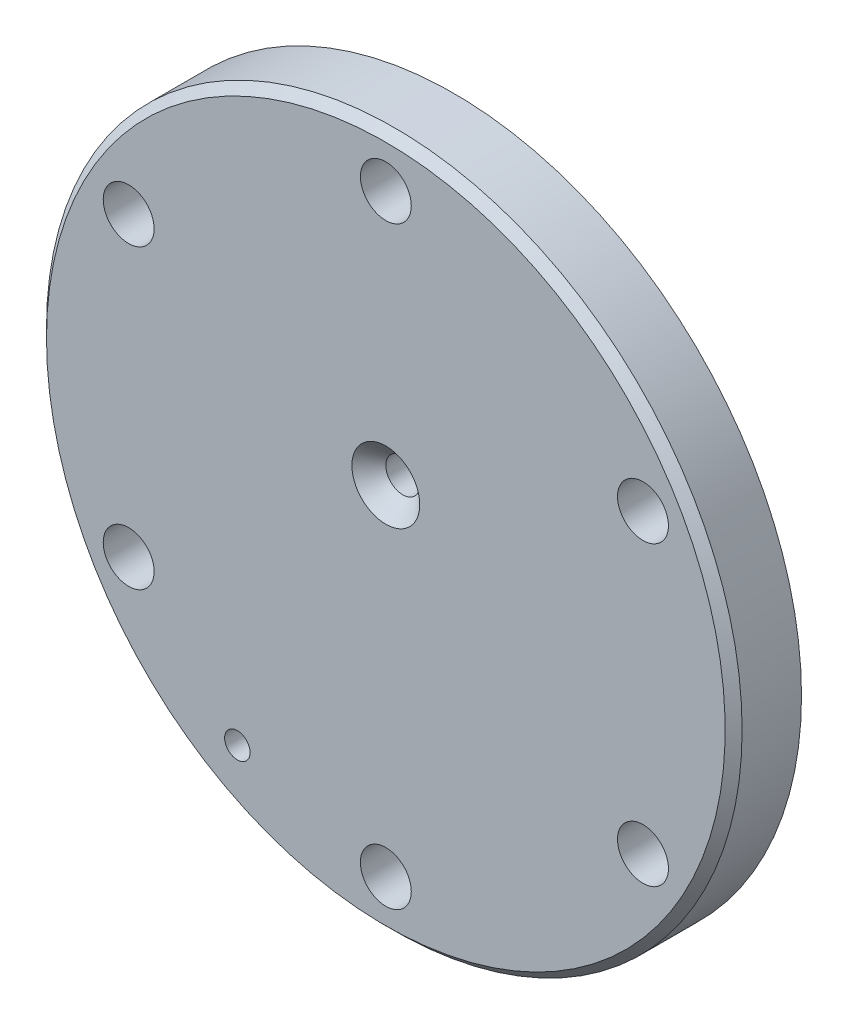
from build123d import *

# Parameters (mm, degrees)
CUT_EXTRUDE1_DEPTH      = 10
CUT_EXTRUDE1_DEPTH_BACK = 59.532042507
SKETCH2_R               = 3
SKETCH2_R_2             = 1.5
SKETCH2_R_3             = 2
CHAMFER1_SIZE           = 1
CHAMFER2_SIZE           = 2


with BuildPart() as part:
    # Sketch1 → Revolve1 (revolve)
    with BuildSketch(Plane(origin=(0, 0, 0), x_dir=(0, 0, -1), z_dir=(1, 0, 0)), mode=Mode.PRIVATE) as revolve1_sk:
        Polygon((0, 0), (0, 24), (-2, 24), (-2, 41), (-10, 41), (-10, 0), align=None)
    revolve(revolve1_sk.sketch.rotate(Axis((0, 0, 25.9375), (0, 0, -1)), 90), axis=Axis((0, 0, 25.9375), (0, 0, -1)))

    # Sketch2 → Cut-Extrude1 (cut, two sides: drawn at the far end of the back side and taken through both)
    with BuildSketch(Plane(origin=(0, 0, 2), x_dir=(-1, 0, 0), z_dir=(0, 0, -1)).offset(-CUT_EXTRUDE1_DEPTH_BACK)):
        with Locations(Location((0, 35, 0), (0, 0, 180))):
            Circle(SKETCH2_R)
        with Locations(Location((30.310889132, 17.5, 0), (0, 0, 180))):
            Circle(SKETCH2_R)
        with Locations(Location((30.310889132, -17.5, 0), (0, 0, 180))):
            Circle(SKETCH2_R)
        with Locations(Location((0, -35, 0), (0, 0, 180))):
            Circle(SKETCH2_R)
        with Locations(Location((-30.310889132, -17.5, 0), (0, 0, 180))):
            Circle(SKETCH2_R)
        with Locations(Location((-30.310889132, 17.5, 0), (0, 0, 180))):
            Circle(SKETCH2_R)
        with Locations(Location((17.5, -30.310889132, 0), (0, 0, 180))):
            Circle(SKETCH2_R_2)
        with Locations(Location((0, 5, 0), (0, 0, 180))):
            Circle(SKETCH2_R_3)
    extrude(amount=CUT_EXTRUDE1_DEPTH + CUT_EXTRUDE1_DEPTH_BACK, mode=Mode.SUBTRACT)

    # Chamfer1
    chamfer1_edges = [part.edges().sort_by_distance(p)[0] for p in [
        (-41, 0, 10),
    ]]
    chamfer(chamfer1_edges, length=CHAMFER1_SIZE)

    # Chamfer2
    chamfer2_edges = [part.edges().sort_by_distance(p)[0] for p in [
        (-2, 5, 10),
    ]]
    chamfer(chamfer2_edges, length=CHAMFER2_SIZE)


solid = part.part
